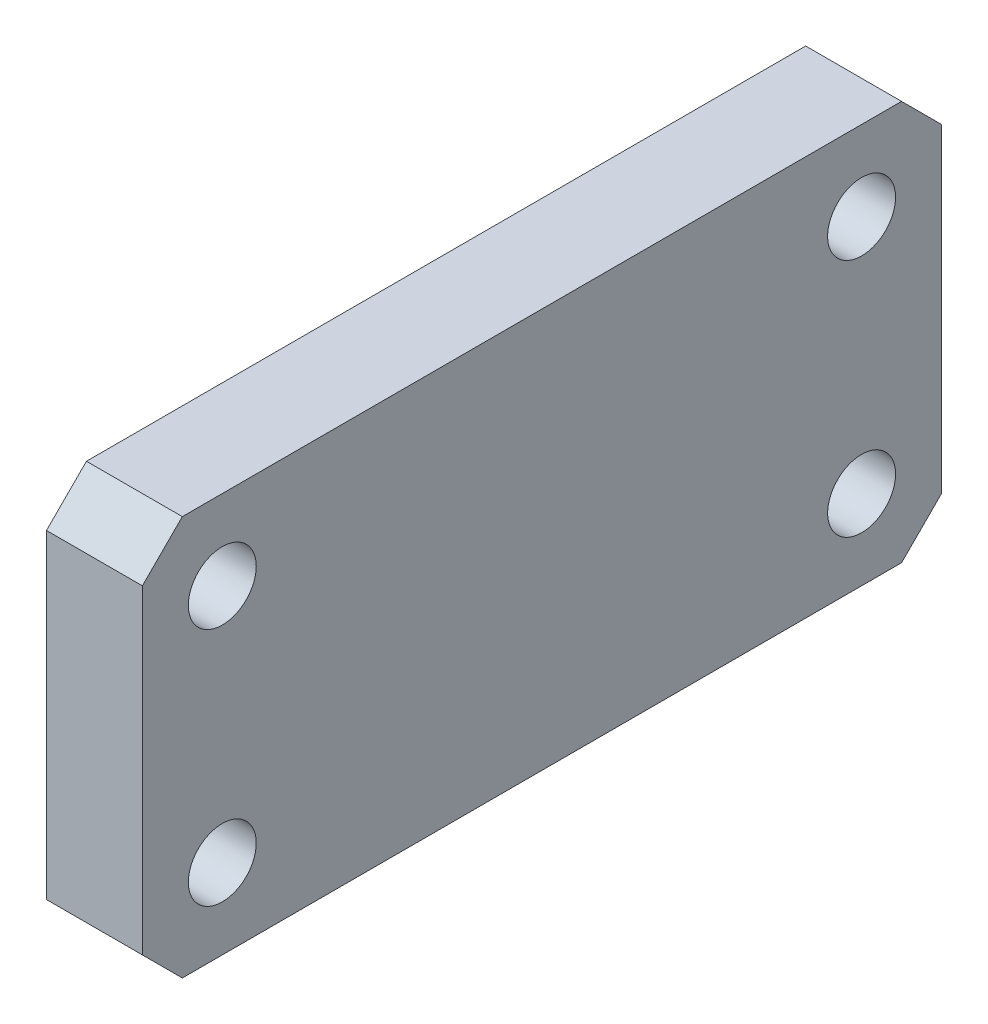
from build123d import *

# Parameters (mm, degrees)
SKETCH_1_W              = 100
SKETCH_1_H              = 50
EXTRUDE_1_DEPTH         = 12
HOLE_WIZARD_8_5_8_5_1_D = 8.5
CHAMFER_1_SIZE          = 5


with BuildPart() as part:
    # 草图1 → 凸台-拉伸1 (new body)
    with BuildSketch(Plane(origin=(0, 0, 0), x_dir=(0, 0, -1), z_dir=(1, 0, 0))):
        Rectangle(SKETCH_1_W, SKETCH_1_H)
    extrude(amount=EXTRUDE_1_DEPTH)

    # Ø8.5 (8.5) 直径孔1 (through all)
    with Locations(Plane(origin=(12, 0, 0), x_dir=(0, 0, -1), z_dir=(1, 0, 0))):
        with Locations((-40, 15), (-40, -15), (40, 15), (40, -15)):
            Hole(HOLE_WIZARD_8_5_8_5_1_D / 2)

    # 倒角1
    chamfer_1_edges = [part.edges().sort_by_distance(p)[0] for p in [
        (6, -25, -50),
        (6, -25, 50),
        (6, 25, 50),
        (6, 25, -50),
    ]]
    chamfer(chamfer_1_edges, length=CHAMFER_1_SIZE)


solid = part.part
